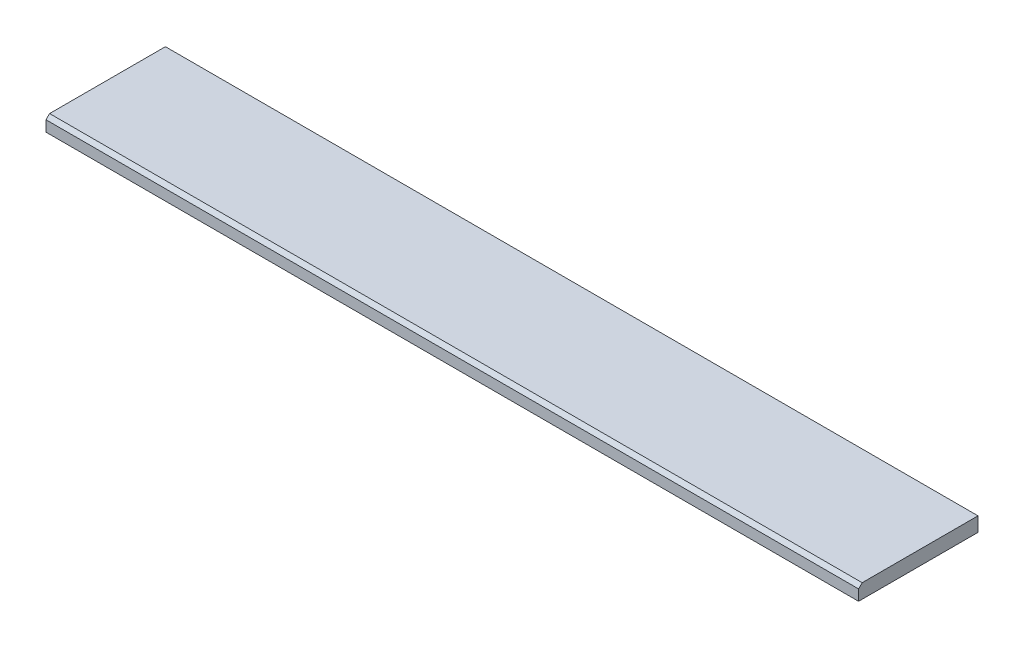
SolidWorks part; units mm, degrees
ref_plane "前视基准面" through (0, 0, 0) normal (0, 0, 1) x (1, 0, 0)
ref_plane "上视基准面" through (0, 0, 0) normal (0, 1, 0) x (1, 0, 0)
ref_plane "右视基准面" through (0, 0, 0) normal (1, 0, 0) x (0, 0, -1)
sketch "草图1" plane through (0, 0, 0) normal (0, 1, 0) x (1, 0, 0)
  line L1 (-1133, -166.5) -> (1133, -166.5)
  line L2 (-1133, -166.5) -> (-1133, 166.5)
  line L3 (-1133, 166.5) -> (1133, 166.5)
  line L4 (1133, -166.5) -> (1133, 166.5)
  line L5 (-1133, -166.5) -> (1133, 166.5) construction
  line L6 (-1133, 166.5) -> (1133, -166.5) construction
  point P0 (0, 0)
  dimension "D1" = 333
  dimension "D2" = 2266
extrude "凸台-拉伸1" add sketch "草图1" along normal blind 40
chamfer "倒角1" distance 10 angle 45 1 edges at (0, 40, 166.5)
